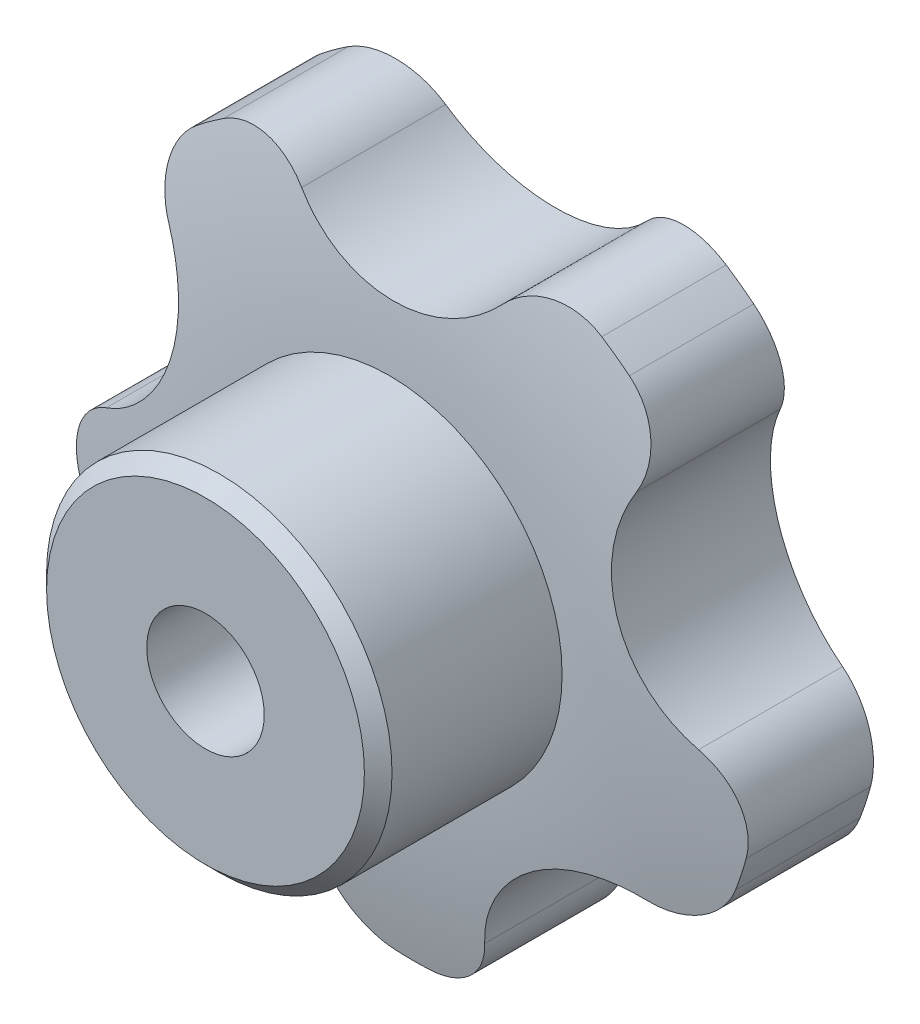
from build123d import *

# Parameters (mm, degrees)
HOLE_WIZARD_M10_1_D      = 8.5
HOLE_WIZARD_M10_1_DEPTH  = 19.5
HOLE_WIZARD_M10_1_TIP    = 2.553657631
SKETCH_4_R               = 10
CUT_EXTRUDE_2_DEPTH      = 36
PATTERN_CIRCULAR_1_COUNT = 5
FILLET_2_R               = 5
CHAMFER_1_SIZE           = 1


with BuildPart() as part:
    # 草图1 → 旋转1 (revolve)
    with BuildSketch(Plane(origin=(0, 0, 0), x_dir=(1, 0, 0), z_dir=(0, 1, 0)), mode=Mode.PRIVATE) as revolve_1_sk:
        with BuildLine():
            Line((25, 24), (25, 15))
            ThreePointArc((25, 15), (18.792676706, 13.838731535), (12.5, 13.30804631))
            Line((12.5, 13.30804631), (12.5, 0))
            Line((12.5, 0), (0, 0))
            Line((0, 0), (0, 26))
            ThreePointArc((0, 26), (12.562319993, 25.778999912), (25, 24))
        make_face()
    revolve(revolve_1_sk.sketch.rotate(Axis((0, 0, -58.488372093), (0, 0, 1)), 180), axis=Axis((0, 0, -58.488372093), (0, 0, 1)))

    # M10 螺纹孔1
    with Locations(Plane.XY):
        with Locations((0, 0)):
            Hole(HOLE_WIZARD_M10_1_D / 2, depth=HOLE_WIZARD_M10_1_DEPTH)
            with Locations((0, 0, -(HOLE_WIZARD_M10_1_DEPTH + HOLE_WIZARD_M10_1_TIP / 2))):  # 118° drill point
                Cone(0, HOLE_WIZARD_M10_1_D / 2, HOLE_WIZARD_M10_1_TIP, mode=Mode.SUBTRACT)

    # 草图4 → 切除-拉伸2 (cut)
    with BuildSketch(Plane.XY):
        with Locations((0, 27)):
            Circle(SKETCH_4_R)
    cut_extrude_2 = extrude(amount=-CUT_EXTRUDE_2_DEPTH, mode=Mode.SUBTRACT)

    # 阵列(圆周)1: 切除-拉伸2 ×5 about axis
    pattern_circular_1_axis = Axis((0, 0, 0), (0, 0, 1))
    for i in range(1, PATTERN_CIRCULAR_1_COUNT):
        add(cut_extrude_2.rotate(pattern_circular_1_axis, i * 360 / PATTERN_CIRCULAR_1_COUNT), mode=Mode.SUBTRACT)

    # 圆角2
    fillet_2_edges = [part.edges().sort_by_distance(p)[0] for p in [
        (-24.946822672, -1.629735742, -19.5),
        (-19.224468863, 15.981858369, -19.5),
        (-9.258962958, 23.222222222, -19.5),
        (9.258962958, 23.222222222, -19.5),
        (-6.159021364, -24.229454303, -19.5),
        (-21.140338131, -13.344890547, -19.5),
        (21.140338131, -13.344890547, -19.5),
        (6.159021364, -24.229454303, -19.5),
        (19.224468863, 15.981858369, -19.5),
        (24.946822672, -1.629735742, -19.5),
    ]]
    fillet(fillet_2_edges, radius=FILLET_2_R)

    # 倒角1
    chamfer_1_edges = [part.edges().sort_by_distance(p)[0] for p in [
        (12.5, 0, 0),
    ]]
    chamfer(chamfer_1_edges, length=CHAMFER_1_SIZE)


solid = part.part
